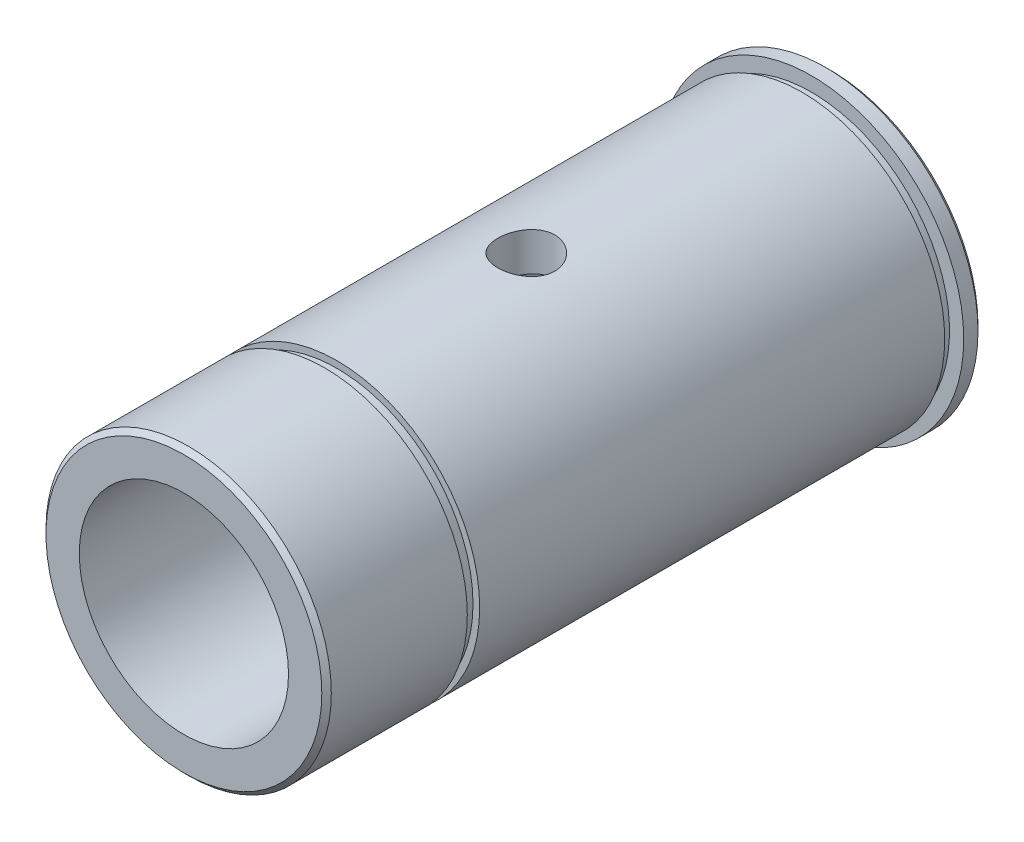
SolidWorks part; units mm, degrees
ref_plane "前视基准面" through (0, 0, 0) normal (0, 0, 1) x (1, 0, 0)
ref_plane "上视基准面" through (0, 0, 0) normal (0, 1, 0) x (1, 0, 0)
ref_plane "右视基准面" through (0, 0, 0) normal (1, 0, 0) x (0, 0, -1)
sketch "草图1" plane through (0, 0, 0) normal (0, 0, 1) x (1, 0, 0)
  circle A0 centre (0, 0) radius 16
  dimension "D1" = 32
extrude "凸台-拉伸1" add sketch "草图1" along normal blind 2
sketch "草图2" plane through (0, 0, 2) normal (0, 0, 1) x (1, 0, 0)
  circle A0 centre (0, 0) radius 15
  dimension "D1" = 30
extrude "凸台-拉伸2" add sketch "草图2" along normal blind 66
sketch "草图3" plane through (0, 0, 0) normal (0, 0, -1) x (-1, 0, 0)
  circle A0 centre (0, 0) radius 9
  dimension "D1" = 18
extrude "切除-拉伸1" cut sketch "草图3" against normal through all
sketch "草图5" plane through (0, 0, 68) normal (0, 0, 1) x (1, 0, 0)
  circle A0 centre (0, 0) radius 11
  dimension "D1" = 22
extrude "切除-拉伸2" cut sketch "草图5" against normal blind 66
cosmetic thread "装饰螺纹线1" parameters "D1"=20, "D2"=24
ref_plane "基准面1" through (0, 15, 0) normal (0, 1, 0) x (1, 0, 0)
sketch "草图8" plane through (0, 15, 0) normal (0, 1, 0) x (1, 0, 0)
  line L0 (-15, -68) -> (15, -68) construction
  line L1 (0, -2) -> (0, -75.071) construction
  line L2 (-15, -2) -> (15, -2) construction
  circle A0 centre (0, -32) radius 3
  dimension "D2" = 6
  dimension "D1" = 36
extrude "切除-拉伸3" cut sketch "草图8" against normal blind 10
sketch "草图9" plane through (0, 0, 0) normal (1, 0, 0) x (0, 0, -1)
  line L0 (-68, 0) -> (13.0117, 0) construction
  line L1 (-51.9, 15) -> (-53.2, 15)
  line L2 (-51.9, 15) -> (-51.9, 14.3)
  line L3 (-51.9, 14.3) -> (-53.2, 14.3)
  line L4 (-53.2, 15) -> (-53.2, 14.3)
  line L5 (-68, 15) -> (-68, -15) construction
  line L6 (19.25, 15) -> (-19.25, 15) construction
  dimension "D1" = 1.3
  dimension "D2" = 14.3
  dimension "D3" = 14.8
revolve "切除-旋转1" cut sketch "草图9" angle 360 about L0
chamfer "倒角1" distance 0.5 angle 45 2 edges at (16, 0, 0) (15, 0, 68)
sketch "草图10" plane through (0, 0, 0) normal (0, 1, 0) x (1, 0, 0)
  line L0 (0, 0) -> (0, -75.6446) construction
  line L1 (-15, -2) -> (-14.5, -2)
  line L2 (-15, -2) -> (-15, -3)
  line L3 (-15, -3) -> (-14.5, -3)
  line L4 (-14.5, -2) -> (-14.5, -3)
  dimension "D1" = 0.5
  dimension "D2" = 1
revolve "切除-旋转2" cut sketch "草图10" angle 360 about L0
